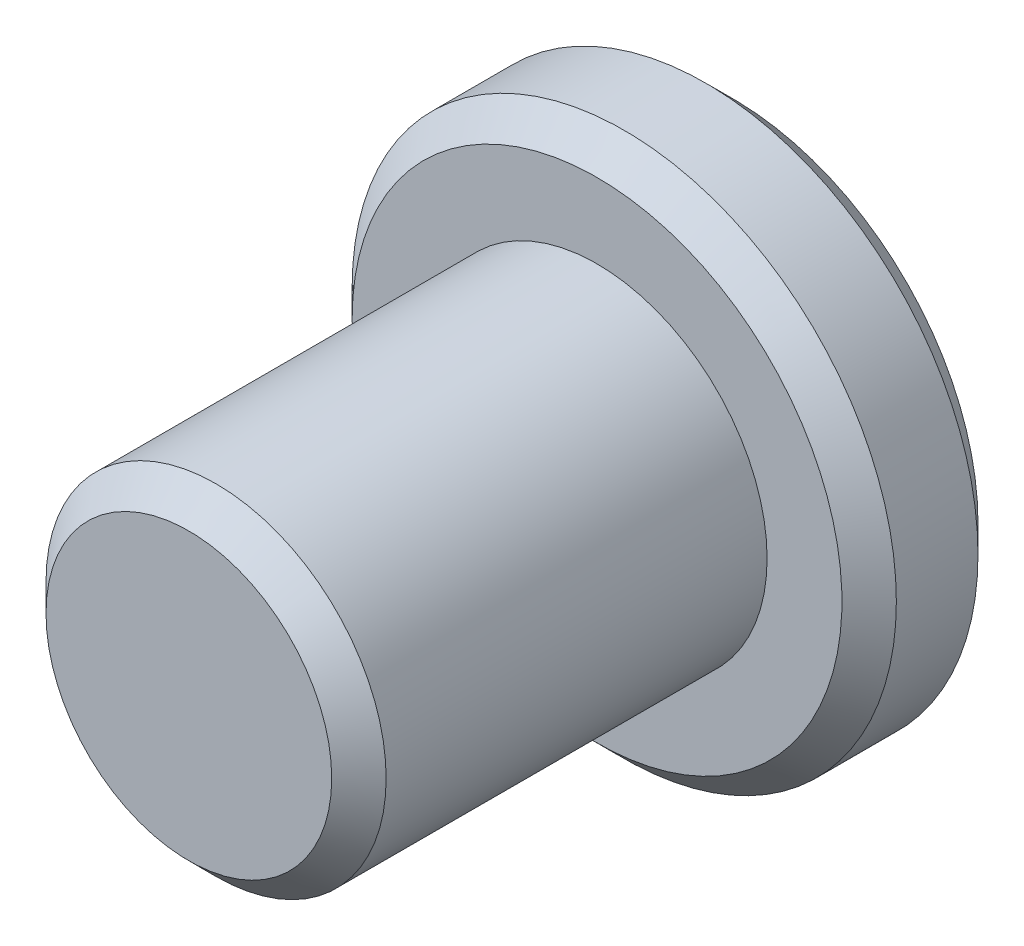
SolidWorks part; units mm, degrees
material "Q235B"
ref_plane "Front Plane" through (0, 0, 0) normal (0, 0, 1) x (1, 0, 0)
ref_plane "Top Plane" through (0, 0, 0) normal (0, 1, 0) x (1, 0, 0)
ref_plane "Right Plane" through (0, 0, 0) normal (1, 0, 0) x (0, 0, -1)
sketch "Sketch1" plane through (0, 0, 0) normal (1, 0, 0) x (0, 0, -1)
  line L0 (0, 0) -> (20, 0) construction
  line L1 (20, 0) -> (20, 10)
  line L2 (20, 10) -> (15, 10)
  line L3 (15, 10) -> (15, 6.25)
  line L4 (15, 6.25) -> (0, 6.25)
  line L7 (0, 6.25) -> (0, 0)
  line L8 (0, 0) -> (20, 0)
  dimension "D2" = 12.5
  dimension "D3" = 20
  dimension "D4" = 5
  dimension "D5" = 15
revolve "Revolve1" add sketch "Sketch1" angle 360 about L0
chamfer "Chamfer1" distance 1 angle 45 3 edges at (10, 0, -20) (10, 0, -15) (6.25, 0, 0)
